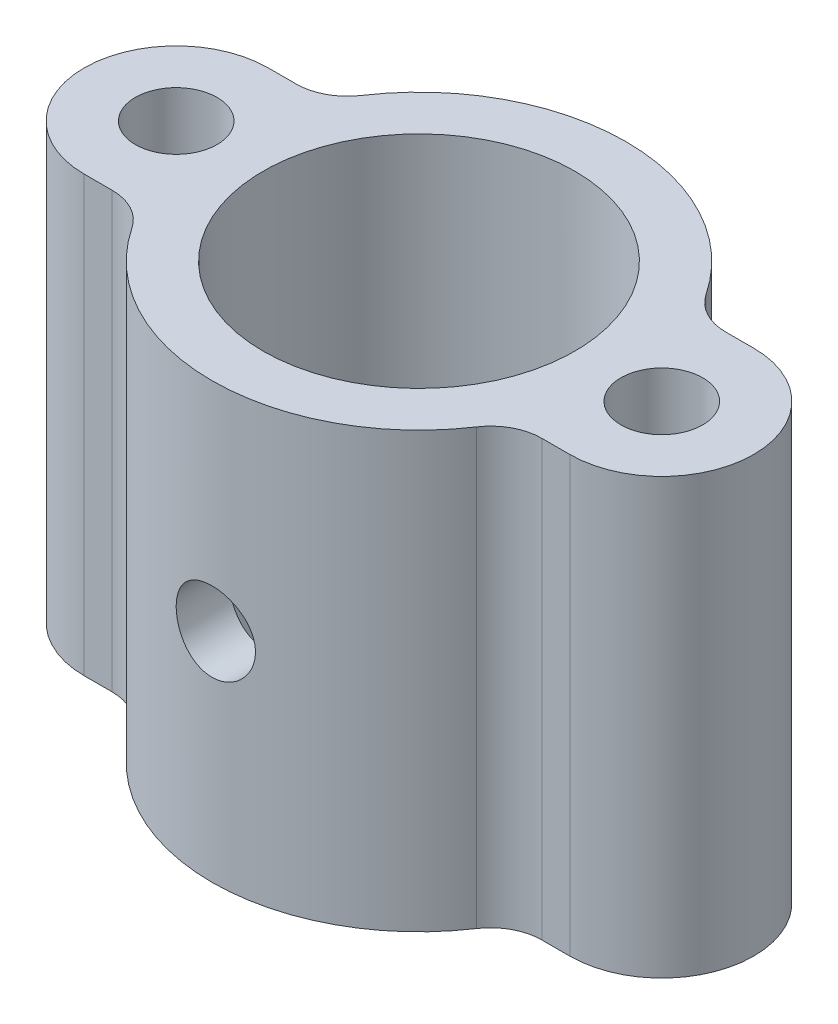
from build123d import *

# Parameters (mm, degrees)
SKETCH_1_R               = 6.1
SKETCH_1_R_2             = 1.6
EXTRUDE_1_DEPTH          = 17
FILLET_1_R               = 2
CUT_EXTRUDE_1_DEPTH      = 23.939485609
CUT_EXTRUDE_1_DEPTH_BACK = 23.939485609
SKETCH_2_R               = 1.55


with BuildPart() as part:
    # 草图1 → 凸台-拉伸1 (new body)
    with BuildSketch(Plane(origin=(0, 0, 0), x_dir=(1, 0, 0), z_dir=(0, 1, 0))):
        with BuildLine():
            Line((9.5, 3.6), (7.256031973, 3.6))
            ThreePointArc((7.256031973, 3.6), (0, 8.1), (-7.256031973, 3.6))
            Line((-7.256031973, 3.6), (-9.5, 3.6))
            ThreePointArc((-9.5, 3.6), (-13.1, 0), (-9.5, -3.6))
            Line((-9.5, -3.6), (-7.256031973, -3.6))
            ThreePointArc((-7.256031973, -3.6), (0, -8.1), (7.256031973, -3.6))
            Line((7.256031973, -3.6), (9.5, -3.6))
            ThreePointArc((9.5, -3.6), (13.1, 0), (9.5, 3.6))
        make_face()
        with Locations(Location((0, 0, 0), (0, 0, 270))):
            Circle(SKETCH_1_R, mode=Mode.SUBTRACT)
        with Locations(Location((9.5, 0, 0), (0, 0, 270))):
            Circle(SKETCH_1_R_2, mode=Mode.SUBTRACT)
        with Locations(Location((-9.5, 0, 0), (0, 0, 90))):
            Circle(SKETCH_1_R_2, mode=Mode.SUBTRACT)
    extrude(amount=EXTRUDE_1_DEPTH)

    # 圆角1
    fillet_1_edges = [part.edges().sort_by_distance(p)[0] for p in [
        (-7.256031973, 8.5, -3.6),
        (7.256031973, 8.5, -3.6),
        (7.256031973, 8.5, 3.6),
        (-7.256031973, 8.5, 3.6),
    ]]
    fillet(fillet_1_edges, radius=FILLET_1_R)

    # 草图2 → 切除-拉伸1 (cut, two sides: drawn at the far end of the back side and taken through both)
    with BuildSketch(Plane.XY.offset(-CUT_EXTRUDE_1_DEPTH_BACK)):
        with Locations((0, 8.5)):
            Circle(SKETCH_2_R)
    extrude(amount=CUT_EXTRUDE_1_DEPTH + CUT_EXTRUDE_1_DEPTH_BACK, mode=Mode.SUBTRACT)


solid = part.part
